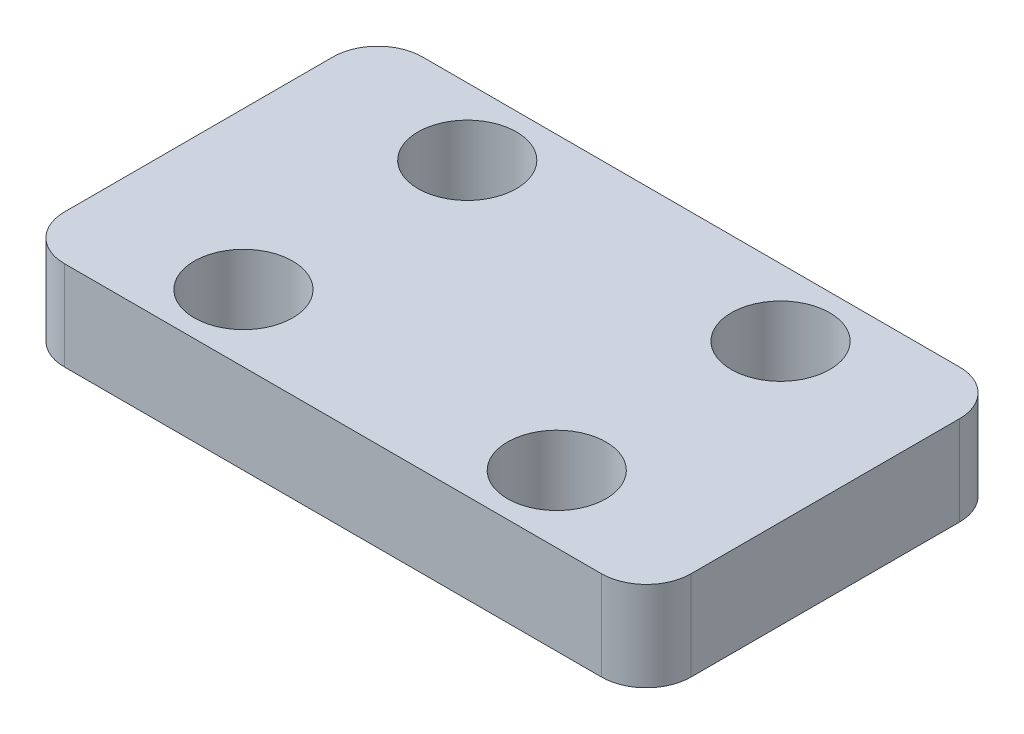
SolidWorks part; units mm, degrees
material "Q235-A"
ref_plane "前视基准面" through (0, 0, 0) normal (0, 0, 1) x (1, 0, 0)
ref_plane "上视基准面" through (0, 0, 0) normal (0, 1, 0) x (1, 0, 0)
ref_plane "右视基准面" through (0, 0, 0) normal (1, 0, 0) x (0, 0, -1)
sketch "草图1" plane through (0, 0, 0) normal (0, 1, 0) x (1, 0, 0)
  line L1 (-35, 20) -> (35, 20)
  line L2 (-35, 20) -> (-35, -20)
  line L3 (-35, -20) -> (35, -20)
  line L4 (35, 20) -> (35, -20)
  line L5 (-35, 20) -> (35, -20) construction
  line L6 (-35, -20) -> (35, 20) construction
  point P0 (0, 0)
  dimension "D1" = 70
  dimension "D2" = 40
extrude "凸台-拉伸1" add sketch "草图1" along normal mid plane 10
hole_wizard "M10 间隙孔1" positions "草图2" profile "草图3" hole size "M10" standard "GB" end condition up to next
sketch "草图2" plane through (0, 5, 0) normal (0, 1, 0) x (1, 0, 0)
  line L0 (0, -5.5) -> (0, 5.5) construction
  line L1 (-5.5, 0) -> (5.5, 0) construction
  point P0 (-17.5, 12.5)
  point P5 (17.5, 12.5)
  point P8 (17.5, -12.5)
  point P9 (-17.5, -12.5)
  dimension "D1" = 35
  dimension "D2" = 25
sketch "草图3" plane through (-17.5, 5, -12.5) normal (1, 0, 0) x (0, 0, 1)
  line L0 (0, 0) -> (0, 10)
  line L1 (0, 10) -> (5.5, 10)
  line L2 (5.5, 10) -> (5.5, 0)
  line L5 (5.5, 0) -> (0, 0)
  line L11 (0, -6.35) -> (0, 107.95) construction
  dimension "通孔孔直径" = 11
  dimension "通孔孔深度" = 10
fillet "圆角1" radius 5 4 edges at (35, 0, 20) (-35, 0, -20) (35, 0, -20) (-35, 0, 20)
